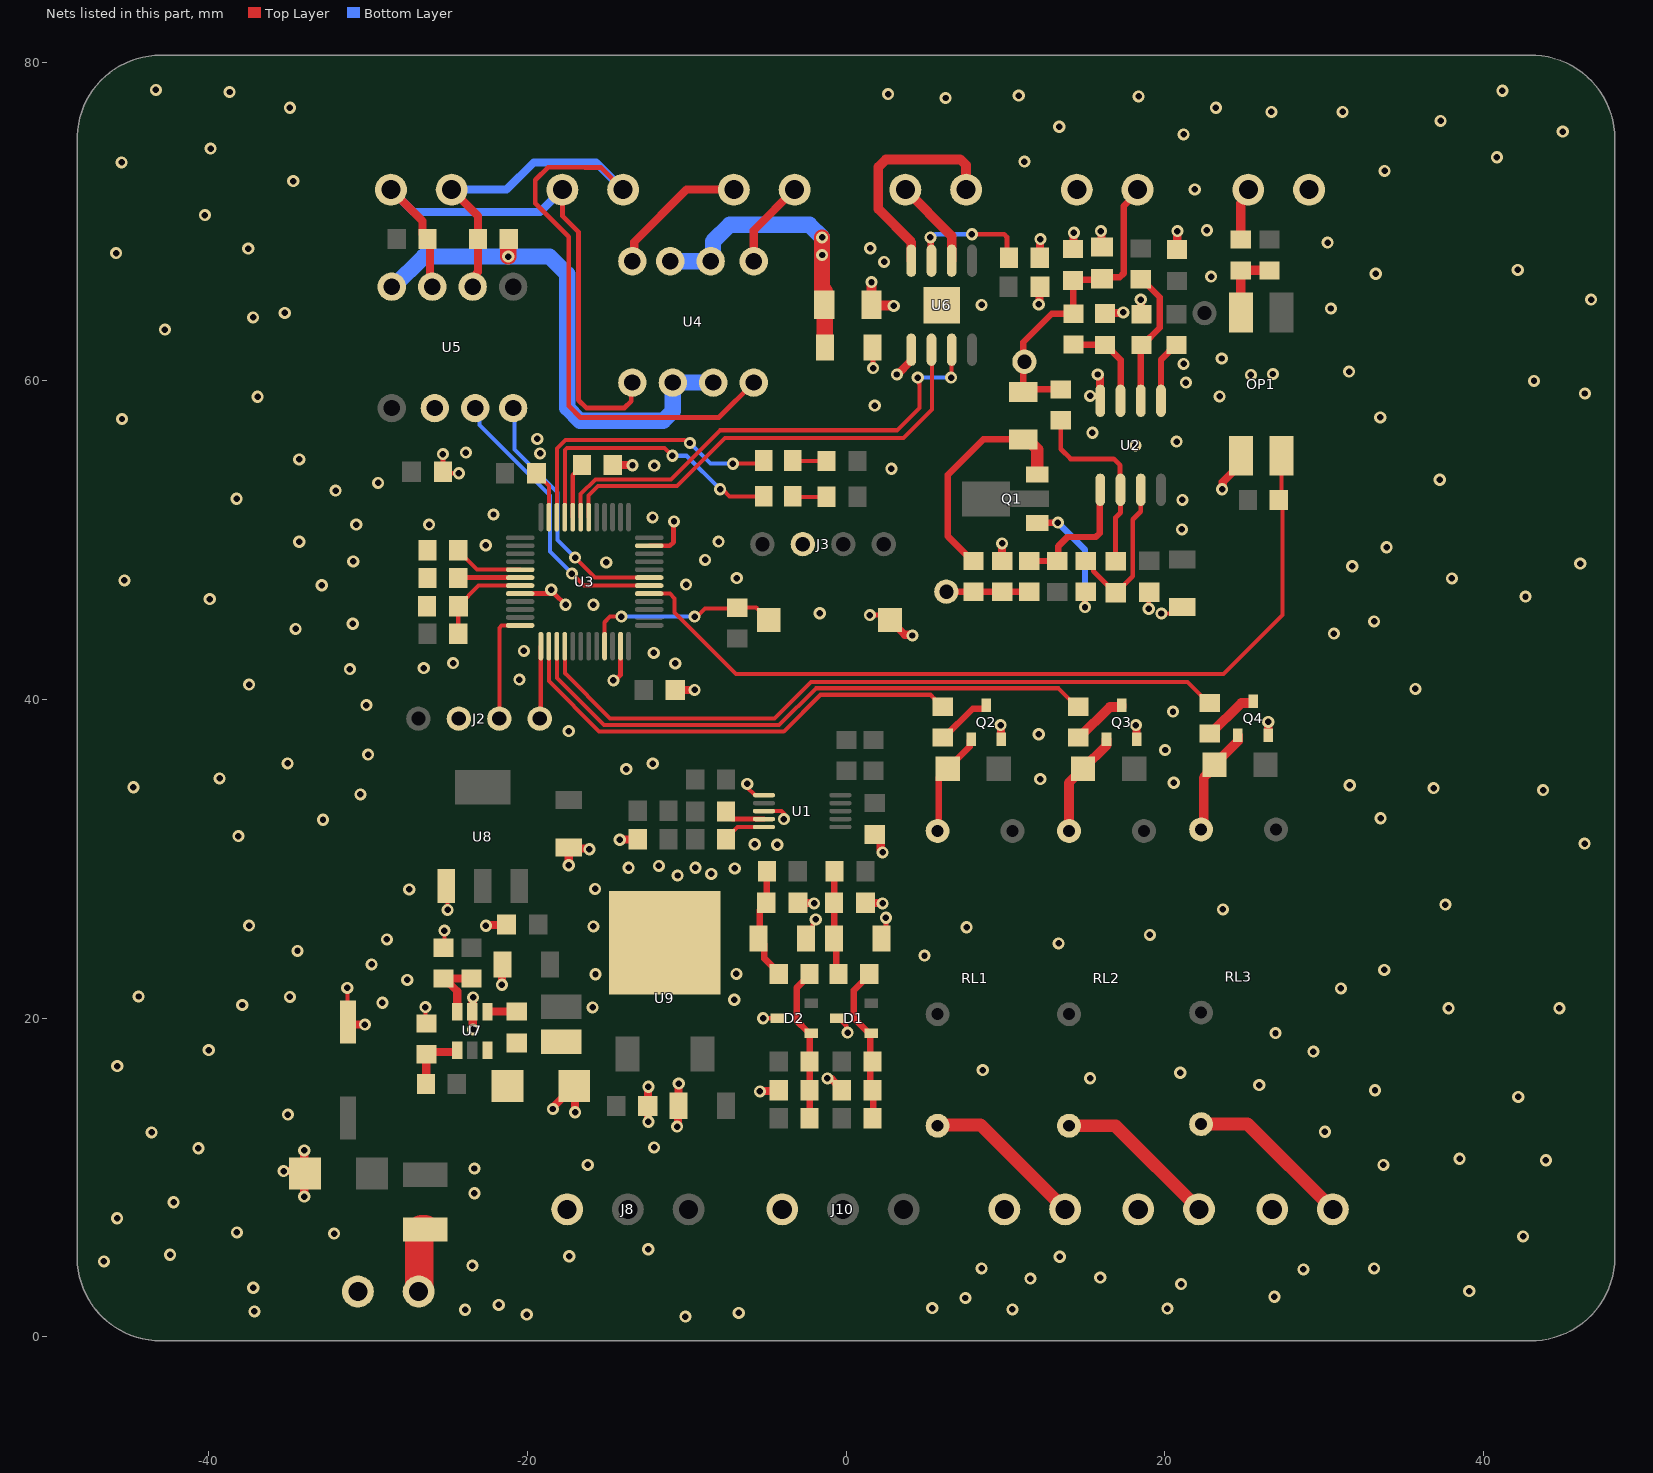
[diagram p0: the nets of this part, all layers, seen from the top]
# Altium PCB MISC82194.PcbDoc (part 2 of 2)
Units mm, origin at the board's own origin, x right, y up, seen from the top; angles counter-clockwise.
Board outline 96.51 x 80.7 mm, 2 copper layers (Top Layer, Bottom Layer); 120 components, 77 nets, 344 pads, 317 vias.
Unrouted connection lines stored in the file: 85.

## Via types
v1: diameter 0.762, hole 0.406, Top Layer to Bottom Layer, 317 vias

## Nets (pads, with @x,y where several pads share a name; then routed paths per layer and width w, separated by ;. In a path a pad name is that pad's centre, name@x,y a point inside that pad or via, vN(x,y) a via of type N, cw(c..) or ccw(c..) an arc to the next point about the centre after c; other vN are vias at no path point) (continued)
DRV-OUT1-1: J6.2 U6.6 | length 5.7
  Top Layer w0.61: J6.2@3.726,72 6.635,69.091 U6.6@6.635,67.544
DRV-OUT1-2: J6.1 U6.8 | length 14.1
  Top Layer w0.61: U6.8@4.095,67.544 4.095,68.705 2.025,70.775 2.025,73.425 2.5,73.9 7.179,73.9 7.536,73.543 J6.1@7.536,72
GND: C2.1 C3.1 C4.1 C5.1 C6.2 C7.1 C8.2 C9.2 C10.2 C11.1 C12.1 C13.1 C14.1 C15.1 C16.1 C17.1 C19.1 C20.1 C21.1 C22.1 C23.1 D1.1 D2.1 D6.1 D7.1 EC1.2 J1.2 J2.3 J3.3 J8.1 J9.1 J10.1 J11.1 J12.1 J13.1 J14.1 OP1.3 Q2.2 Q3.2 Q4.2 R2.2 R13.1 R17.2 R18.2 R22.2 R23.2 R24.2 R25.1 R28.1 R36.1 R37.1 R48.2 R49.1 S1.1 U1.1 U1.3 U2.4 U3.8 U3.23 U3.35 U3.47 U5.3 U6.1 U6.9 U7.2 U8.1 U9.2 | length 86.1
  Top Layer w0.254: v1(-31.3,21.9) -31.3,19.8 EC1.2@-31.25,19.75 ; v1(-26.4,20.7) -26.4,19.74 R49.1@-26.325,19.665 ; R48.2@-25.258,24.416 -25.2,24.474 v1(-25.2,25.5) ; U8.1@-25.1,28.3 -25,28.2 v1(-25,26.8) ; C13.1@-19.419,54.2 -19.419,54.165 -18.65,53.396 U3.47@-18.65,51.45 ; v1(-6.2,34.7) -6.2,34.49 -5.71,34 U1.1@-5.15,34 ; U1.3@-5.15,33 -4.049,33 -3.9,32.851 v1(-3.9,32.5) ; v1(19,45.7) 19,46.709 C3.1@19.025,46.735 ; v1(19.8,45.4) 20.68,45.4 C2.1@21.1,45.82
  Top Layer w0.3: U3.8@-20.45,46.65 -18.304,46.65 v1(-17.602,45.949) ; U3.35@-12.35,49.65 -11.056,49.65 -10.82,49.886 -10.82,51.156 v1(-10.795,51.181)
  Top Layer w0.305: v1(-25.3,55.4) C9.2@-25.3,54.3 -25.2,54.2 v1(-24.3,54.2) ; v1(-14.6,41.2) -14.5,41.2 -14.15,41.55 U3.23@-14.15,43.35 ; v1(-5.2,20) D2.1@-4.325,20 ; C15.1@-2.5,25 -2.087,25.413 -2.087,25.889 -1.9,26.076 v1(-1.9,26.2) ; D1.1@-0.575,20 -0.45,20 0.013,19.537 0.013,19.187 v1(0.1,19.1) ; v1(1.5,45.3) S1.1@2.91,45.3 ; C8.2@1.65,62.1 1.7,62.05 v1(1.7,60.8) ; C11.1@2.23,25 2.5,25.27 v1(2.5,26.3)
  Top Layer w0.508: v1(-35.3,10.4) -34.086,10.4 D7.1@-34,10.314 ; v1(-34,8.8) -34,10.209 D7.1@-33.948,10.262 D7.1@-34,10.314 ; v1(-34,11.7) D7.1@-34,10.314 ; EC1.2@-31.25,19.75 -31.1,19.6 v1(-30.2,19.6) ; v1(-23.4,19.3) -23.425,19.325 -23.425,20.375 U7.2@-23.45,20.4 -23.425,20.425 -23.425,21.275 v1(-23.4,21.3) ; v1(-22.6,25.8) -22.563,25.837 -21.337,25.837 C21.1@-21.3,25.875 ; v1(-21.6,22.1) -21.581,22.119 -21.581,23.351 C19.1@-21.563,23.37 ; v1(-18.4,14.3) -18.351,14.349 -18.351,14.439 D6.1@-17.052,15.738 -17,15.686 v1(-17,14.1) ; v1(-17.4,29.6) C20.1@-17.4,30.7 -17.349,30.649 -16.149,30.649 v1(-16.1,30.6) ; R25.1@-14.635,54.725 -14.622,54.713 -13.413,54.713 v1(-13.4,54.7) ; v1(-14.2,31.2) -14.187,31.213 -13.078,31.213 R17.2@-13.065,31.225 ; v1(-12.4,13.5) -12.421,13.521 -12.421,14.475 C23.1@-12.441,14.496 -12.421,14.517 -12.421,15.679 v1(-12.4,15.7) ; C14.1@-10.719,40.6 v1(-9.5,40.6) ; v1(-10.6,13.2) -10.551,13.249 -10.551,14.449 C22.1@-10.5,14.5 v1(-10.5,15.9) ; v1(-5.4,15.4) -5.363,15.437 -4.253,15.437 R37.1@-4.215,15.475 ; C16.1@-3.019,27.25 -2.994,27.225 -2.025,27.225 v1(-2,27.2) ; v1(-1.163,16.218) -1.114,16.17 -0.897,16.17 -0.465,15.738 R36.1@-0.465,15.475 ; C12.1@1.231,27.25 1.256,27.225 2.275,27.225 v1(2.3,27.2) ; C7.1@1.8,31.519 1.835,31.519 2.181,31.173 2.181,30.588 2.3,30.469 v1(2.3,30.4) ; S1.1@2.91,45.3 2.905,45.295 2.905,44.847 3.685,44.067 4.117,44.067 v1(4.166,44.018) ; v1(3.2,60.4) 3.225,60.4 4.095,61.27 U6.1@4.095,61.956 ; v1(9.7,38.4) 9.725,38.375 9.725,37.525 Q2.2@9.75,37.5 ; R18.2@9.801,48.7 v1(9.8,49.8) ; v1(12.1,64.8) 12.141,64.841 12.141,65.859 C17.1@12.181,65.9 ; R28.1@12.165,67.725 12.183,67.743 12.183,68.883 v1(12.2,68.9) ; C6.2@14.25,68.277 14.275,68.302 14.275,69.275 v1(14.3,69.3) ; v1(15.8,60.4) 15.8,60.331 15.941,60.191 15.941,58.769 U2.4@15.96,58.75 ; v1(16,69.4) 16.037,69.363 16.037,68.428 R13.1@16.075,68.391 ; C5.1@16.25,64.231 16.284,64.266 17.366,64.266 v1(17.4,64.3) ; v1(18.2,38.4) 18.225,38.375 18.225,37.525 Q3.2@18.25,37.5 ; v1(18.5,65.1) 18.525,65.075 18.525,64.206 R2.2@18.551,64.18 ; C4.1@20.775,68.25 20.788,68.262 20.788,69.388 v1(20.8,69.4) ; v1(23.6,53.2) 23.649,53.249 23.649,53.649 24.8,54.8 OP1.3@24.8,55.3 ; Q4.2@26.5,37.75 v1(26.5,38.6)
  Top Layer w0.61: v1(1.6,66.2) 1.604,66.196 1.604,64.787 R22.2@1.608,64.783 1.661,64.729 2.971,64.729 v1(3,64.7)
  other v1: -10.084,1.27 -20.041,1.397 -6.731,1.499 -37.135,1.6 -23.901,1.702 10.439,1.727 20.168,1.778 5.41,1.803 -21.793,2.007 7.493,2.438 26.889,2.514 39.116,2.87 -37.199,3.079 21.034,3.311 11.576,3.657 15.959,3.714 28.704,4.233 8.509,4.293 33.147,4.293 -23.444,4.47 -46.572,4.738 13.411,5.029 -17.374,5.055 -42.418,5.156 -12.408,5.494 42.494,6.299 -32.131,6.477 -38.227,6.553 -45.745,7.442 -42.197,8.451 -23.317,9.017 -23.317,10.566 -16.205,10.795 33.728,10.788 43.929,11.086 38.506,11.176 -40.64,11.836 -12.04,11.887 -43.586,12.827 30.06,12.871 -35.027,13.945 42.189,15.062 33.202,15.479 25.933,15.799 15.324,16.228 20.976,16.574 8.585,16.747 -45.741,16.993 29.338,17.901 -39.997,18 26.956,19.069 37.821,20.625 44.78,20.625 -15.9,20.676 -37.897,20.828 -29.101,20.967 -7.01,21.158 -34.9,21.336 -44.399,21.361 31.064,21.869 -27.534,22.403 -15.723,22.758 -6.883,22.784 33.779,23.033 -29.778,23.373 4.928,23.927 -34.425,24.226 13.34,24.689 -28.819,24.948 19.078,25.223 7.569,25.705 -15.85,25.756 -37.465,25.806 23.66,26.824 37.617,27.127 -27.411,28.088 -15.748,28.118 -10.566,28.956 -8.458,29.058 -6.986,29.398 -13.64,29.439 -9.449,29.439 -11.743,29.557 -4.316,30.883 -5.73,30.919 46.355,30.963 -38.132,31.428 -32.825,32.455 33.548,32.549 -30.479,34.043 43.748,34.312 36.881,34.442 -44.729,34.493 31.615,34.62 20.574,34.773 12.192,35.001 -39.319,35.052 -13.792,35.636 -12.127,35.975 -35.052,35.992 -29.989,36.539 20.025,36.832 12.096,37.823 -17.399,38.024 20.523,39.243 -30.099,39.649 35.738,40.665 -37.46,40.94 -20.497,41.252 -31.14,41.91 -26.504,41.97 -10.719,42.266 -24.663,42.291 -12.065,42.926 -20.218,43.053 30.617,44.133 -34.55,44.432 -30.96,44.756 33.147,44.907 -1.651,45.415 -15.85,45.949 -39.929,46.304 42.647,46.457 -18.502,46.891 -32.902,47.169 -10.033,47.219 -45.288,47.473 38.024,47.6 -6.858,47.625 31.77,48.361 46.081,48.527 -15.044,48.606 -30.93,48.669 -8.839,48.768 33.934,49.555 -22.606,49.682 -34.314,49.905 -8.001,49.911 21.082,50.673 -30.734,50.978 -26.162,50.978 -12.141,51.435 -22.123,51.613 21.118,52.527 -38.252,52.603 -32.029,53.111 -29.362,53.594 37.262,53.797 2.845,54.483 -12.03,54.681 -34.314,55.069 -19.202,55.448 -23.851,55.499 18.164,55.951 20.752,56.185 -19.38,56.363 15.469,56.744 -45.441,57.607 33.528,57.709 1.803,58.445 -36.932,59.004 23.444,59.03 15.316,59.055 46.38,59.207 21.336,59.893 43.18,59.995 25.414,60.373 26.788,60.43 31.578,60.581 21.184,61.062 23.583,61.404 -42.748,63.221 -37.211,63.983 -35.23,64.262 30.429,64.541 8.509,64.77 46.761,65.1 22.911,66.548 33.249,66.726 42.161,66.963 2.388,67.462 -45.816,68.021 -37.516,68.301 1.524,68.326 30.226,68.682 22.647,69.454 -40.234,70.409 21.888,72.022 -34.696,72.542 33.807,73.177 -45.466,73.711 11.201,73.762 40.853,74.035 -39.878,74.574 21.184,75.463 44.983,75.641 13.386,75.946 37.317,76.311 26.695,76.886 31.166,76.886 -34.9,77.14 23.216,77.14 6.249,77.754 18.364,77.851 10.846,77.902 2.642,78.003 -38.684,78.13 41.199,78.207 -43.307,78.257
LED1: LED1.2 U3.45 | length 18
  Top Layer w0.254: U3.45@-17.65,51.45 -17.65,55.651 -17.501,55.8 -11.4,55.8 v1(-10.9,55.3) ; v1(-7.9,53.2) -7.763,53.2 -7.313,52.75 LED1.2@-5.169,52.75
  Bottom Layer w0.254: v1(-10.9,55.3) -10,55.3 v1(-7.9,53.2)
LED2: LED2.2 U3.46 | length 18.2
  Top Layer w0.254: U3.46@-18.15,51.45 -18.15,55.75 -17.6,56.3 -10.137,56.3 -9.937,56.1 v1(-9.8,56.1) ; v1(-7.1,54.8) -5.369,54.8 LED2.2@-5.169,55
  Bottom Layer w0.254: v1(-9.8,56.1) -8.5,54.8 v1(-7.1,54.8)
NetC1_1: C1.1 R5.2 U2.7 | length 9.9
  Top Layer w0.305: R5.2@15.114,48.7 15.533,48.281 15.533,48.057 16.443,47.148 16.89,46.7 16.96,46.7 18,47.74 18,51.3 18.5,51.8 U2.7@18.5,53.162
  Top Layer w0.762: R5.2@15.051,48.7 R5.2@15.068,48.717
NetC1_2: C1.2 R1.2 U2.6 | length 12.1
  Top Layer w0.305: R1.2@13.475,57.535 13.475,55.725 14.1,55.1 16.8,55.1 17.2,54.7 17.2,53.192 U2.6@17.23,53.162 17.23,51.73 16.925,51.425 C1.2@16.925,48.681
NetC5_2: C5.2 R10.1 U2.3 | length 5.9
  Top Layer w0.406: R10.1@14.275,62.285 14.293,62.267 16.233,62.267 C5.2@16.25,62.25 16.314,62.25 17.23,61.333 U2.3@17.23,58.75
NetC6_1: C6.1 J1.1 R1.1 R9.2 R10.2 R13.2 T2.1 | length 20.5
  Top Layer w0.406: R1.1@13.475,59.465 11.275,59.465 R9.2@11.117,59.308 11.117,62.417 12.915,64.215 R10.2@14.275,64.215 14.275,66.27 C6.1@14.25,66.296 14.307,66.353 16.018,66.353 16.165,66.5 17.18,66.5 17.418,66.738 17.418,70.965 18.298,71.845 J1.1@18.298,72
NetC10_1: C10.1 R29.1 U3.7 | length 6.2
  Top Layer w0.254: R29.1@-24.335,44.125 -24.335,45.834 C10.1@-24.319,45.85 -24.319,45.885 -23.054,47.15 U3.7@-20.45,47.15
NetC11_2: C11.2 C12.2 R31.2 R32.1 | length 6.6
  Top Layer w0.406: R32.1@-0.715,29.225 -0.733,29.207 -0.733,27.267 C12.2@-0.75,27.25 C11.2@-0.75,25 -0.608,24.858 -0.608,22.918 R31.2@-0.465,22.775
NetC15_2: C15.2 C16.2 R34.2 R35.1 | length 7.2
  Top Layer w0.406: R35.1@-4.965,29.225 -4.983,29.207 -4.983,27.267 C16.2@-5,27.25 -5,27.186 -5.4,26.786 -5.4,25.08 C15.2@-5.48,25 -5.118,24.638 -5.118,23.742 -4.584,23.207 -4.215,22.839 R34.2@-4.215,22.775
NetC18_1: C18.1 D6.2 L1.1 U7.6
NetC18_2: C18.2 U7.1 | length 1.8
  Top Layer w0.508: U7.1@-22.5,20.4 -22.487,20.413 -20.68,20.413 C18.2@-20.668,20.425
NetD1_3: D1.3 R26.1 R30.2 R31.1 R36.2 | length 10.1
  Top Layer w0.406: R31.1@1.465,22.775 1.465,22.712 0.5,21.747 0.5,20 1.45,19.05 D1.3@1.575,19.05 1.52,18.995 1.52,15.62 1.7,15.44 1.7,13.759 R30.2@1.665,13.725
NetD2_3: D2.3 R27.1 R33.2 R34.1 R37.2 | length 9.9
  Top Layer w0.406: R33.2@-2.285,13.725 R37.2@-2.285,15.475 R27.1@-2.285,17.275 -2.285,18.953 D2.3@-2.188,19.05 ; R34.1@-2.285,22.775 -2.285,22.712 -3.1,21.897 -3.1,19.85 -2.397,19.147 -2.3,19.05 D2.3@-2.175,19.05
NetD3_1: D3.1 Q2.3 RL1.2 | length 6.6
  Top Layer w0.406: RL1.2@5.75,31.75 5.82,31.82 5.82,35.097 7.753,37.031 7.753,37.403 Q2.3@7.85,37.5
NetD4_1: D4.1 Q3.3 RL2.2 | length 6.7
  Top Layer w0.61: RL2.2@14,31.75 14,34.778 D4.1@14.879,35.656 16.345,37.123 16.345,37.495 Q3.3@16.35,37.5
NetD5_1: D5.1 Q4.3 RL3.2 | length 6.9
  Top Layer w0.61: RL3.2@22.288,31.847 22.451,32.01 22.451,35.092 22.671,35.313 22.671,35.449 23.586,36.363 23.586,36.386 24.6,37.4 Q4.3@24.6,37.75
NetLED1_1: LED1.1 R39.1 | length 2.1
  Top Layer w0.254: LED1.1@-3.33,52.75 -3.305,52.725 R39.1@-1.215,52.725
NetLED2_1: LED2.1 R40.1 | length 2.1
  Top Layer w0.254: LED2.1@-3.33,55 -3.305,54.975 R40.1@-1.215,54.975
NetOP1_2: OP1.2 R42.1 R43.2 | length 4.4
  Top Layer w0.61: OP1.2@24.8,64.3 24.775,64.325 R43.2@24.775,66.935 R42.1@26.575,66.935
NetQ1_1: Q1.1 R5.1 | length 8.3
  Top Layer w0.406: Q1.1@12.007,51.076 12.019,51.088 13.288,51.088 v1(13.3,51.1) ; v1(15,45.8) 15,46.719 R5.1@15.051,46.77
  Bottom Layer w0.406: v1(13.3,51.1) 15,49.4 v1(15,45.8)
NetQ1_2: Q1.2 R9.1 R14.1 | length 14.5
  Top Layer w0.406: R14.1@8,48.7 7.937,48.7 6.4,50.237 6.4,54.1 8.628,56.328 R9.1@11.117,56.328
  Top Layer w0.762: R9.1@11.117,56.328 11.382,56.328 12.007,55.703 Q1.2@12.007,54.124
NetQ2_1: Q2.1 R44.1 | length 3.6
  Top Layer w0.406: R44.1@6.075,37.61 6.139,37.61 7.957,39.428 8.703,39.428 8.8,39.525 Q2.1@8.8,39.65
NetQ3_1: Q3.1 R45.1 | length 3.6
  Top Layer w0.61: R45.1@14.575,37.61 14.639,37.61 16.559,39.53 17.295,39.53 17.3,39.535 Q3.1@17.3,39.65
NetQ4_1: Q4.1 R46.1 | length 3.6
  Top Layer w0.61: R46.1@22.825,37.86 22.889,37.86 24.809,39.78 25.545,39.78 25.55,39.785 Q4.1@25.55,39.9
NetR2_1: R2.1 R3.2 U2.2 | length 8.7
  Top Layer w0.406: U2.2@18.5,58.75 18.5,62.199 R2.1@18.551,62.25 18.614,62.25 19.7,63.336 19.7,65.245 18.564,66.382 R3.2@18.5,66.382
NetR7_2: R7.2 U2.1 | length 3.9
  Top Layer w0.406: U2.1@19.77,58.75 19.77,61.333 20.687,62.25 R7.2@20.75,62.25
NetR12_2: R12.2 U1.4 | length 2.6
  Top Layer w0.305: R12.2@-7.535,32.975 -7.535,32.919 -7.116,32.5 U1.4@-5.15,32.5
NetR14_2: R14.2 R15.2 R18.1 T3.1 | length 5.2
  Top Layer w0.406: T3.1@6.3,46.77 R14.2@8,46.77 R18.1@9.801,46.77 R15.2@11.5,46.77
NetR15_1: R15.1 R19.1 U2.5 | length 8.4
  Top Layer w0.406: R15.1@11.5,48.7 11.506,48.694 13.256,48.694 R19.1@13.263,48.687 13.33,48.755 13.33,49.63 13.9,50.2 15.683,50.2 15.921,50.438 15.921,53.123 U2.5@15.96,53.162
NetR16_2: R16.2 U1.5 | length 2.7
  Top Layer w0.254: R16.2@-7.535,31.225 -7.535,31.288 -6.823,32 U1.5@-5.15,32
NetR23_1: R23.1 U3.5 | length 4.4
  Top Layer w0.254: R23.1@-24.335,49.375 -24.335,49.312 -23.173,48.15 U3.5@-20.45,48.15
NetR24_1: R24.1 U3.6 | length 3.9
  Top Layer w0.305: R24.1@-24.335,47.625 -24.31,47.65 U3.6@-20.45,47.65
NetR25_2: R25.2 U3.44 | length 3.5
  Top Layer w0.254: U3.44@-17.15,51.45 -17.15,54.077 -16.565,54.662 R25.2@-16.565,54.725
NetR28_2: R28.2 U6.7 | length 7.8
  Top Layer w0.305: v1(7.9,69.2) 9.921,69.2 10.1,69.021 10.1,67.86 R28.2@10.235,67.725
  Top Layer w0.406: v1(5.3,69) 5.332,68.967 5.332,67.577 U6.7@5.365,67.544
  Bottom Layer w0.305: v1(5.3,69) 5.424,69 5.624,69.2 v1(7.9,69.2)
NetR47_2: R47.2 R48.1 U7.3 | length 4.2
  Top Layer w0.508: R48.1@-25.258,22.486 R48.1@-25.194,22.486 ; U7.3@-24.4,20.4 -24.4,21.692 R48.1@-25.194,22.486 ; R47.2@-23.508,22.486 R48.1@-25.194,22.486
NetR49_2: R49.2 R50.1 U7.4 | length 3.9
  Top Layer w0.508: R50.1@-26.365,15.875 -26.345,15.895 -26.345,17.715 R49.2@-26.325,17.735 -26.193,17.867 -24.471,17.867 -24.4,17.938 U7.4@-24.4,18
P-485-A: J7.2 U4.1 | length 8.9
  Top Layer w0.508: U4.1@-13.41,67.51 -13.291,67.629 -13.291,68.709 -10,72 J7.2@-7.036,72
P-485-B: J7.1 U4.4 | length 5.6
  Top Layer w0.508: U4.4@-5.79,67.51 -5.79,69.436 J7.1@-3.226,72 ; U4.4@-5.547,67.173 U4.4@-5.5,67.22
PE: C8.1 R22.1 U4.2 U4.3 | length 19.5
  Top Layer w1.016: v1(-1.5,69) v1(-1.5,67.9) -1.5,65.794 -1.33,65.624 C8.1@-1.33,62.1
  Bottom Layer w1.016: U4.2@-11.033,67.51 U4.3@-8.493,67.51 -8.347,67.656 -8.347,68.753 -7.3,69.8 -2.3,69.8 v1(-1.5,69) v1(-1.5,67.9)
PWM1-1: U3.42 U6.2 | length 28.9
  Top Layer w0.254: U3.42@-16.15,51.45 -16.15,52.817 -15.567,53.4 -10.6,53.4 -7.594,56.406 3.606,56.406 5.4,58.2 5.4,61.921 U6.2@5.365,61.956
PWM1-2: U3.43 U6.3 | length 30.7
  Top Layer w0.254: U3.43@-16.65,51.45 -16.65,52.892 -15.735,53.806 -10.994,53.806 -7.9,56.9 3.2,56.9 4.6,58.3 4.6,59.797 4.597,59.8 4.597,60.103 v1(4.5,60.2) ; v1(6.6,60.2) 6.618,60.217 6.618,61.938 U6.3@6.635,61.956
  Bottom Layer w0.254: v1(4.5,60.2) v1(6.6,60.2)
R-GND: R21.1 U4.6 U4.7 U5.5 | length 33.3
  Top Layer w1.016: v1(-21.2,67.8) -21.2,68.87 R21.1@-21.17,68.9
  Bottom Layer w1.016: U5.5@-28.51,65.91 -28.404,65.91 -26.514,67.8 v1(-21.2,67.8) -18.6,67.8 -17.5,66.7 -17.5,58.3 -16.7,57.5 -11.465,57.5 -10.87,58.095 U4.7@-10.87,59.89 U4.6@-8.33,59.89
RL1: R44.2 U3.14 | length 29.5
  Top Layer w0.254: U3.14@-18.65,43.35 -18.65,41.15 -15.494,37.994 -3.906,37.994 -1.6,40.3 5.316,40.3 5.567,40.048 5.567,39.985 6.012,39.54 R44.2@6.075,39.54
RL2: R45.2 U3.15 | length 37.4
  Top Layer w0.254: U3.15@-18.15,43.35 -18.15,41.35 -15.2,38.4 -4.2,38.4 -1.894,40.706 13.346,40.706 14.512,39.54 R45.2@14.575,39.54
RL3: R46.2 U3.16 | length 44.9
  Top Layer w0.254: U3.16@-17.65,43.35 -17.65,41.65 -14.807,38.807 -4.493,38.807 -2.187,41.113 21.439,41.113 22.762,39.79 R46.2@22.825,39.79
RLOUT1: J11.2 RL1.4 | length 10.3
  Top Layer w0.813: RL1.4@5.75,13.25 5.7,13.3 8.45,13.3 J11.2@13.75,8
RLOUT2: J12.2 RL2.4 | length 10.3
  Top Layer w0.813: RL2.4@14,13.25 16.905,13.25 J12.2@22.155,8
RLOUT3: J13.2 RL3.4 | length 10.5
  Top Layer w0.813: RL3.4@22.288,13.347 25.213,13.347 J13.2@30.56,8
RS-485A: J4.2 J5.2 R20.1 U4.8 U5.6 | length 37.7
  Top Layer w0.305: J4.2@-17.798,72 -17.798,70.351 -16.8,69.353 -16.8,58.8 -16.3,58.3 -13.9,58.3 -13.478,58.722 -13.478,59.822 U4.8@-13.41,59.89
  Top Layer w0.508: J5.2@-28.56,72 -26.587,70.027 -26.587,69.217 R20.1@-26.27,68.9 -26.12,68.75 -26.12,66.06 U5.6@-25.97,65.91
  Bottom Layer w0.508: J5.2@-28.56,72 -27.154,70.594 -19.204,70.594 J4.2@-17.798,72 ; U4.8@-13.31,59.94 U4.8@-13.31,60.01
RS-485B: J4.1 J5.1 R21.2 U4.5 U5.7 | length 53.4
  Top Layer w0.305: J4.1@-13.988,72 -15.388,73.4 -16.4,73.4 -16.406,73.406 -18.7,73.406 -19.5,72.606 -19.5,71.138 -17.4,69.038 -17.4,58.432 -16.668,57.7 -7.98,57.7 U4.5@-5.79,59.89
  Top Layer w0.508: J5.1@-24.75,72 -23.1,70.35 -23.1,66.843 -23.187,66.756 -23.187,66.153 U5.7@-23.43,65.91
  Bottom Layer w0.508: J5.1@-24.75,72 -21.3,72 -19.6,73.7 -15.688,73.7 J4.1@-13.988,72
RX: J2.1 U3.13 | length 4.6
  Top Layer w0.254: J2.1@-19.22,38.8 -19.159,38.861 -19.159,43.341 U3.13@-19.15,43.35
RX-485: U3.31 U5.1 | length 16.3
  Top Layer w0.254: v1(-17,48.91) -15.74,47.65 U3.31@-12.35,47.65
  Bottom Layer w0.254: U5.1@-20.8,58.497 -20.8,55.7 -18.1,53 -18.1,50.01 v1(-17,48.91)
SW1: R38.1 S1.2 U3.21 | length 12.5
  Top Layer w0.254: U3.21@-15.15,43.35 -15.15,44.85 -14.8,45.2 v1(-14.1,45.2) ; v1(-9.5,45.2) -9.363,45.2 -8.863,45.7 -6.891,45.7 R38.1@-6.825,45.765 -5.633,45.765 S1.2@-4.851,44.983
  Bottom Layer w0.254: v1(-14.1,45.2) v1(-9.5,45.2)
TTL-IN1: J14.2 R43.1 | length 3.3
  Top Layer w0.61: R43.1@24.775,68.865 24.775,71.148 25.25,71.624 J14.2@25.25,72
TTLMCU-IN1: OP1.4 R41.1 U3.29 | length 53.8
  Top Layer w0.254: U3.29@-12.35,46.65 -11.05,46.65 -10.75,46.35 -10.75,45.45 -6.9,41.6 23.707,41.6 27.4,45.293 R41.1@27.4,52.298 ; R41.1@27.165,52.525 27.34,52.7 OP1.4@27.34,55.3
TX: J2.2 U3.12 | length 7.1
  Top Layer w0.254: J2.2@-21.76,38.8 -21.76,44.501 -21.611,44.65 U3.12@-20.45,44.65
TX-485: U3.30 U5.2 | length 18.2
  Top Layer w0.254: v1(-17.2,47.9) -16.45,47.15 U3.30@-12.35,47.15
  Bottom Layer w0.254: U5.2@-23,58.522 -23,57.217 -18.583,52.8 -18.583,49.283 v1(-17.2,47.9)
VIN: F1.1 J9.2 | length 4.2
  Top Layer w1.8: J9.2@-26.822,2.845 -26.784,2.883 -26.784,6.601 -26.646,6.739 F1.1@-26.419,6.739
pads on no net: U3.1 U3.2 U3.3 U3.4 U3.10 U3.11 U3.17 U3.18 U3.19 U3.20 U3.27 U3.28 U3.32 U3.33 U3.38 U3.39 U3.40

## Polygon pours and split planes (outlines as drawn)
GND on Bottom Layer "GND_L02_P000" (solid, remove dead copper, pour order 0): 1,59.5 -1.25,57.25 -24.25,57.25 -24.75,57.75 -24.75,59 -25,59.25 -26.5,59.25 -27,58.75 -27,57.25 -28,56.25 -49.414,56.25 -49.414,-0.75 48.237,-0.75 48.237,81 1.5,81 1,80.5
GND on Bottom Layer "GND_L02_P003" (solid, remove dead copper, pour order 3): -33.766,55.423 -32.995,56.194 -32.995,81.534 -35.281,83.82 -46.965,83.82 -49.301,81.483 -49.276,81.458 -49.276,57.277 -47.422,55.423
GND on Top Layer "GND_L01_P001" (solid, remove dead copper, pour order 1): 1.01,59.505 -1.24,57.255 -24.24,57.255 -24.74,57.755 -24.74,59.005 -24.99,59.255 -26.49,59.255 -26.99,58.755 -26.99,57.255 -27.99,56.255 -47.758,56.255 -48.031,55.982 -48.031,-0.995 48.237,-0.995 48.237,80.505 1.01,80.505
GND on Top Layer "GND_L01_P004" (solid, remove dead copper, pour order 4): -33.766,55.194 -32.995,55.965 -32.995,81.305 -35.281,83.591 -46.965,83.591 -49.301,81.255 -49.276,81.229 -49.276,57.048 -47.422,55.194

## Keep-outs
Keep-Out Layer:
  circle w0.3: c43,40.025 r1.75
  circle w0.3: c43,52.525 r1.75
  circle w0.3: c43,27.525 r1.75
  circle w0.3: c-43,27.525 r1.75
  circle w0.3: c-43,52.525 r1.75
  circle w0.3: c-43,40.03 r1.75
  lines w0.508: -48,4.648 -48,75.336 ; -48,5 ccw(c-43,5) -43,0 43.231,0 ; -48,75.188 cw(c-43,75.188) -43,80.188 43.205,80.188 ; 43,0.004 ccw(c43,5.004) 48,5.004 ; 43,80.184 cw(c43,75.184) 48,75.184 48,4.674

## Other copper
Top Layer:
  region net 12V: -9.8,18.9 -9.8,16.6 -8.4,15.2 -8.4,13.5 -8.1,13.2 -6.7,13.2 -6.4,13.5 -6.4,18.2 -7.1,18.9
  region net 3.3V: -23.4,27.2 -23.6,27.4 -23.6,29.5 -24,29.9 -27.5,29.9 -28.1,30.5 -28.1,35.9 -27.5,36.5 -16.7,36.5 -16,35.8 -16,33.2 -16.6,32.6 -19.1,32.6 -19.5,32.2 -19.5,30 -21.3,30 -22,29.3 -22,27.4 -22.2,27.2
  region net 5.7V: -19.2,24.4 -20.1,25.3 -20.1,26.8 -21,27.7 -21,29.5 -19.2,29.5 -16.7,27 -16.7,20.4 -19.1,20.4 -19.2,20.5
  region net NetC18_1: -22.8,16.3 -21.6,15.1 -20.4,15.1 -20.4,16.5 -19.3,17.6 -16.8,17.6 -16.5,17.9 -16.5,19.2 -16.6,19.3 -21.1,19.3 -21.8,18.6 -22.8,18.6
  region net 24V: -23.8,18.5 -23.8,17.2 -25,16 -25,13.5 -23.1,13.5 -23.1,18.5

## Silkscreen, mask and mechanical layers (free items; w line width, h text height)
Top Overlay:
  text "3.3v" at -6.916,47.516 h0.8
  text "DIO" at -0.82,47.516 h0.8
  text "CLK" at 1.746,47.516 h0.8
  text "GND" at -3.639,47.466 h0.8
  text "3.3v" at -28.607,36.213 h0.8
  text "GND" at -25.001,36.188 h0.8
  text "TX" at -22.156,36.163 h0.8
  text "RX" at -19.895,36.163 h0.8